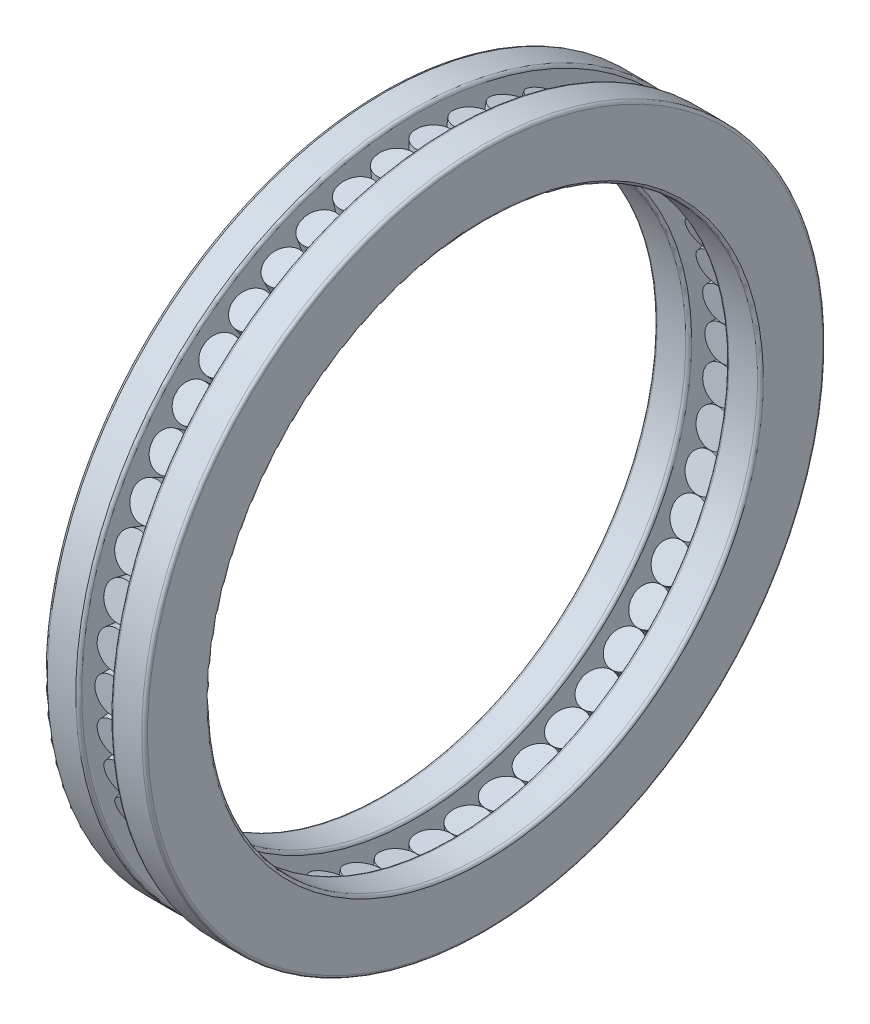
SolidWorks part; units mm, degrees
ref_plane "Front" through (0, 0, 0) normal (0, 0, 1) x (1, 0, 0)
ref_plane "Top" through (0, 0, 0) normal (0, 1, 0) x (1, 0, 0)
ref_plane "Right" through (0, 0, 0) normal (1, 0, 0) x (0, 0, -1)
sketch "Sketch1" plane through (-7.03, 10.47, 0) normal (0, 0, 1) x (0, 1, 0)
  line L0 (-10.47, 18.1553) -> (-10.47, -14.7153) construction
  line L1 (-27.97, 45.97) -> (-20.47, 45.97) construction
  line L2 (-183.97, -7.03) -> (-150.47, -7.03)
  line L3 (-183.97, -7.03) -> (-183.97, 10.6366)
  line L4 (-183.97, 10.6366) -> (-150.47, 10.6366)
  line L5 (-150.47, -7.03) -> (-150.47, 10.6366)
revolve "Revolve1" add sketch "Sketch1" angle 360 about L0
sketch "Sketch2" plane through (1.5709, -3.0291, 0) normal (0, 0, 1) x (0, -1, 0)
  line L0 (-19.5753, 7.2625) -> (17.0395, 7.2625) construction
  line L2 (-168.1541, 7.2625) -> (-168.1541, 16.1958)
  line L4 (-168.1541, 16.1958) -> (-151.4041, 16.1958)
  line L5 (-151.4041, 16.1958) -> (-151.4041, 7.2625)
  line L7 (-168.1541, 7.2625) -> (-151.4041, 7.2625)
revolve "Revolve2" add sketch "Sketch2" angle 360 about L0
sketch "Sketch3" plane through (-8.783, 8.717, 0) normal (0, 0, 1) x (0, 1, 0)
  line L0 (-8.717, 6.8297) -> (-8.717, -6.8957) construction
  line L1 (-183.717, -26.4497) -> (-150.217, -26.4497)
  line L2 (-183.717, -26.4497) -> (-183.717, -44.1163)
  line L3 (-183.717, -44.1163) -> (-150.217, -44.1163)
  line L4 (-150.217, -26.4497) -> (-150.217, -44.1163)
  line L5 (139.658, -26.5497) -> (156.408, -26.5497) construction
revolve "Revolve3" add sketch "Sketch3" angle 360 about L0
pattern_circular "Circular-Pattern1" count 52 over 360 about axis through (0, 0, 0) along (1, 0, 0) of "Revolve2"
fillet "Fillet1" radius 1.5 8 edges at (0, -173.5, 0) (-17.6667, -173.5, 0) (-17.6667, -140, 0) (0, -140, 0) (17.6667, -141.5, 0) (35.3333, -141.5, 0) (35.3333, -175, 0) (17.6667, -175, 0)
equation "\"D3@Sketch1\" = \"H@Sketch1\" / 3"
equation "\"D1@Sketch2\" = \"H@Sketch1\" / 3 + 0.2"
equation "\"D4@Sketch2\" = \"D1@Sketch2\" / 2 - 0.1"
equation "\"D3@Sketch2\" =  ( \"DD1@Sketch1\" - \"XD@Sketch1\" )  / 4"
equation "\"D2@Sketch2\" = \"XD@Sketch1\" / 2 +  ( \"DD1@Sketch1\" - \"XD@Sketch1\" )  / 8"
equation "\"D1@Circular-Pattern1\" = int ( 3.14 / atn (  ( \"D1@Sketch2\" / 2 )  / sqr (  ( \"D2@Sketch2\" * \"D2@Sketch2\" )  -  ( \"D1@Sketch2\" / 2 )  *  ( \"D1@Sketch2\" / 2 )  )  )  )"
equation "\"D2@Sketch3\" = \"H@Sketch1\" / 3"
